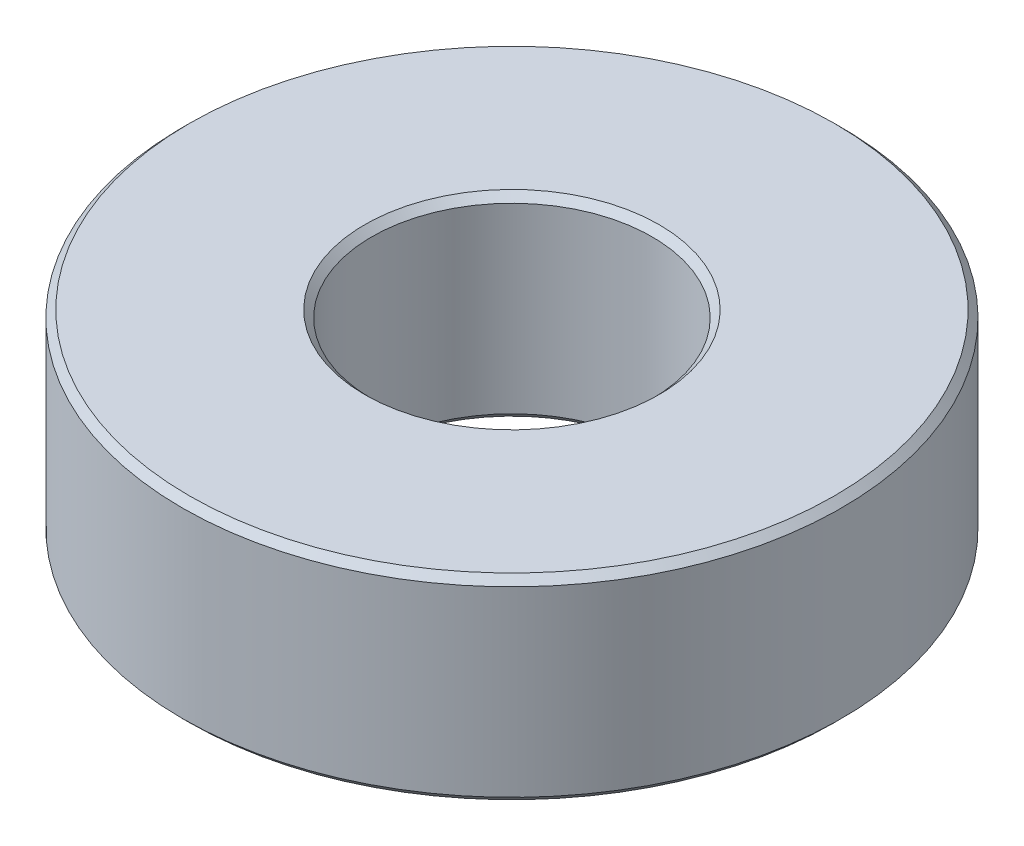
SolidWorks part; units mm, degrees
ref_plane "前视" through (0, 0, 0) normal (0, 0, 1) x (1, 0, 0)
ref_plane "上视" through (0, 0, 0) normal (0, 1, 0) x (1, 0, 0)
ref_plane "右视" through (0, 0, 0) normal (1, 0, 0) x (0, 0, -1)
sketch "草图1" plane through (0, 0, 0) normal (0, 1, 0) x (1, 0, 0)
  circle A0 centre (0, 0) radius 23.5
  circle A1 centre (0, 0) radius 10
extrude "拉伸1" add sketch "草图1" along normal blind 14
chamfer "倒角1" distance 0.5 angle 45 4 edges at (0, 0, 10) (0, 0, 23.5) (0, 14, 23.5) (0, 14, 10)
